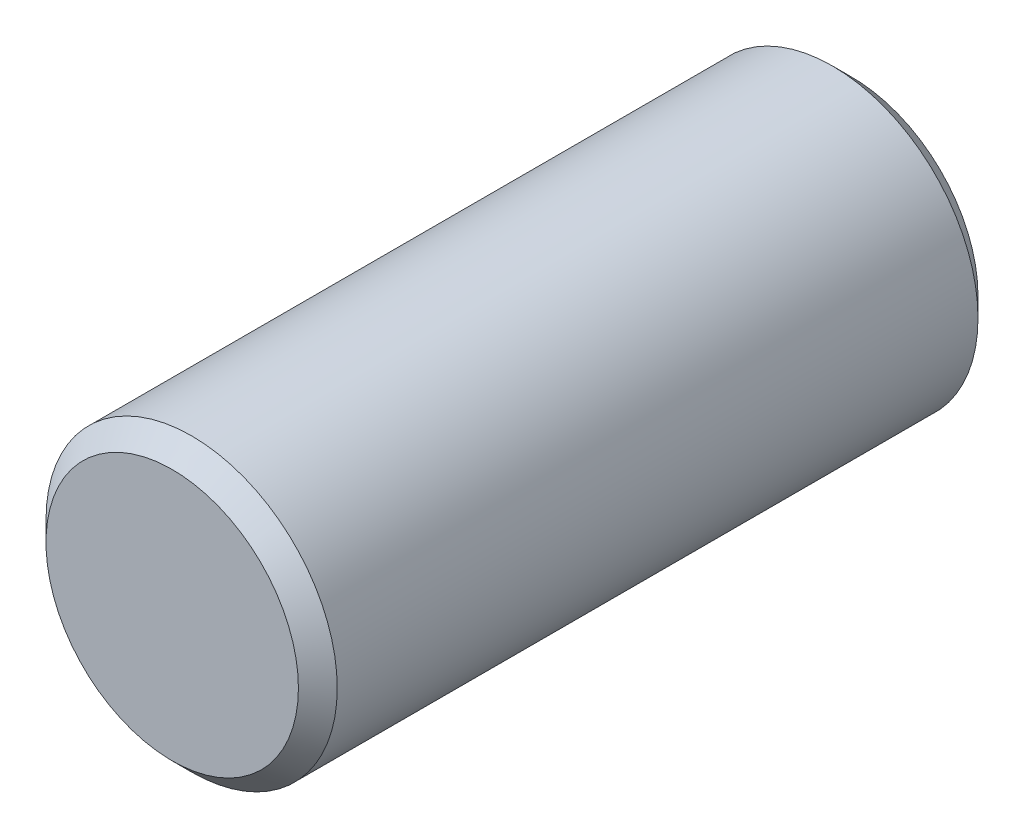
from build123d import *

# Parameters (mm, degrees)
SKETCH2_R           = 1.5
BOSS_EXTRUDE2_DEPTH = 7
CHAMFER1_SIZE       = 0.2


with BuildPart() as part:
    # Sketch2 → Boss-Extrude2 (new body)
    with BuildSketch(Plane.XY):
        with Locations((-3.05913896, 37.271986881)):
            Circle(SKETCH2_R)
    extrude(amount=BOSS_EXTRUDE2_DEPTH)

    # Chamfer1
    chamfer1_edges = [part.edges().sort_by_distance(p)[0] for p in [
        (-4.55913896, 37.271986881, 0),
        (-4.55913896, 37.271986881, 7),
    ]]
    chamfer(chamfer1_edges, length=CHAMFER1_SIZE)


solid = part.part
